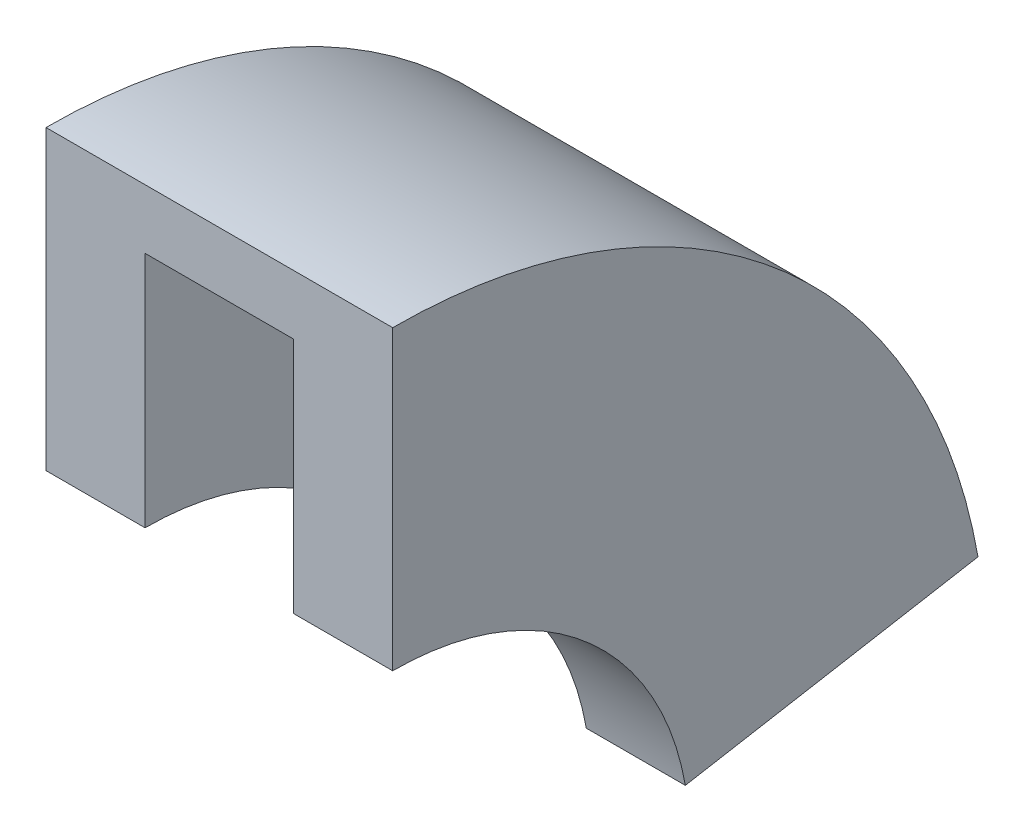
from build123d import *

# Parameters (mm, degrees)
REVOLVE1_ANGLE                 = 80
SKETCH3_R                      = 7.5
BOSS_EXTRUDE1_DEPTH            = 10
SHELL3_T                       = -5
CUT_EXTRUDE1_REACH             = 176.812
SKETCH4_R                      = 15
CUT_EXTRUDE1_DIRECTION_2_REACH = 176.812


with BuildPart() as part:
    # Sketch1 → Revolve1 (revolve)
    with BuildSketch(Plane.XY):
        Polygon((-0.136394071, 58.716551136), (19.863605929, 58.716551136), (19.863605929, 118.716551136), (-50.136394071, 118.716551136), (-50.136394071, 58.716551136), (-30.136394071, 58.716551136), (-30.136394071, 106.716551136), (-0.136394071, 106.716551136), align=None)
    revolve(axis=Axis((39.541450035, -1.283448864, 0), (-1, 0, 0)), revolution_arc=REVOLVE1_ANGLE)

    # Sketch3 → Boss-Extrude1 (add)
    with BuildSketch(Plane.ZY.offset(50.136394071)):
        with Locations((-48.209070726, 56.16988437)):
            Circle(SKETCH3_R)
    extrude(amount=BOSS_EXTRUDE1_DEPTH)

    # Shell3
    shell3_openings = [part.faces().sort_by_distance(p)[0] for p in [
        (-60.136394071, 56.16988437, -48.209070726),
    ]]
    offset(amount=SHELL3_T, openings=shell3_openings, kind=Kind.INTERSECTION)

    # Sketch4 → Cut-Extrude1 (cut, up to next)
    with BuildSketch(Plane(origin=(-30.136394071, 0, 0), x_dir=(0, 0, -1), z_dir=(1, 0, 0)), mode=Mode.PRIVATE) as cut_extrude1_sk1:
        with Locations(Location((52.708583994, 61.532195472, 0), (0, 0, 270))):
            Circle(SKETCH4_R)
    cut_extrude1_tool1 = extrude(cut_extrude1_sk1.sketch, amount=-CUT_EXTRUDE1_REACH, mode=Mode.PRIVATE) & part.part
    add(cut_extrude1_tool1.solids().sort_by_distance((-30.136394, 61.532195, -52.708584))[0], mode=Mode.SUBTRACT)

    # Sketch4 → Cut-Extrude1 direction 2 (cut, up to next)
    with BuildSketch(Plane(origin=(-30.136394071, 0, 0), x_dir=(0, 0, -1), z_dir=(1, 0, 0)), mode=Mode.PRIVATE) as cut_extrude1_direction_2_sk1:
        with Locations(Location((52.708583994, 61.532195472, 0), (0, 0, 270))):
            Circle(SKETCH4_R)
    cut_extrude1_direction_2_tool1 = extrude(cut_extrude1_direction_2_sk1.sketch, amount=CUT_EXTRUDE1_DIRECTION_2_REACH, mode=Mode.PRIVATE) & part.part
    add(cut_extrude1_direction_2_tool1.solids().sort_by_distance((-30.136394, 61.532195, -52.708584))[0], mode=Mode.SUBTRACT)


solid = part.part
